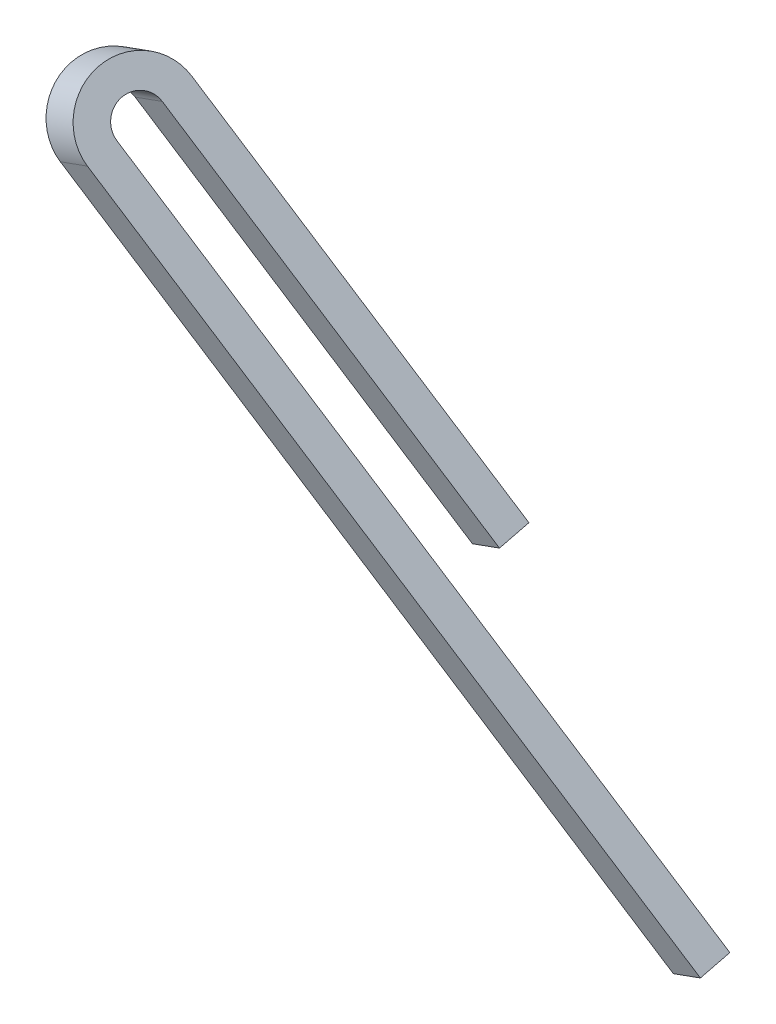
from build123d import *

# Parameters (mm, degrees)
EXTRUDE_1_DEPTH = 34


with BuildPart() as part:
    # 草图2 → 拉伸-薄壁1 (new, symmetric)
    with BuildSketch(Plane(origin=(290.969985959, -860.871008049, 2246.011610274), x_dir=(-0.12461162955889699, -0.382773527459934, 0.9153995676504089), z_dir=(0.8091108722091485, 0.49479707812616053, 0.3170417132661968))):
        with BuildLine():
            Line((0, 712.5), (0, -209.427913233))
            ThreePointArc((0, -209.427913233), (-62, -271.427913233), (-124, -209.427913233))
            Line((-124, -209.427913233), (-124, 297.758706857))
            Line((-124, 297.758706857), (-89, 297.758706857))
            Line((-89, 297.758706857), (-89, -209.427913233))
            ThreePointArc((-89, -209.427913233), (-62, -236.427913233), (-35, -209.427913233))
            Line((-35, -209.427913233), (-35, 712.5))
            Line((-35, 712.5), (0, 712.5))
        make_face()
    extrude(amount=EXTRUDE_1_DEPTH, both=True)


solid = part.part
